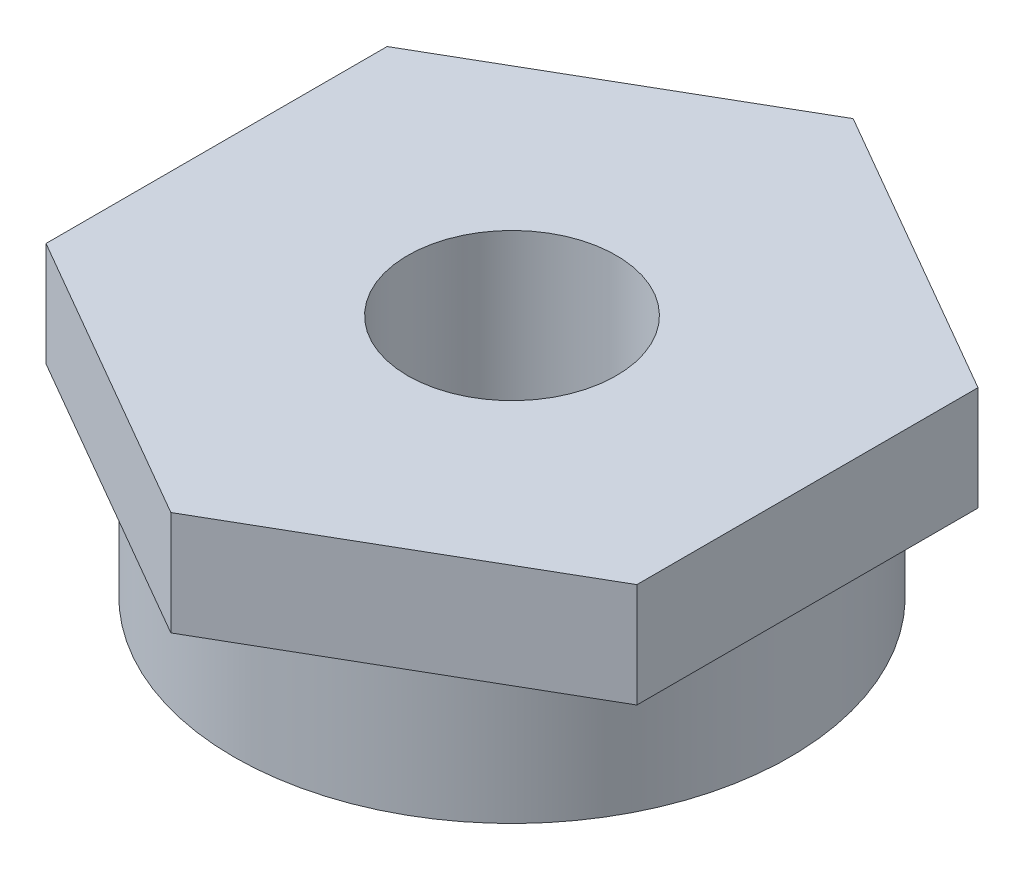
SolidWorks part; units mm, degrees
material "Q235A"
ref_plane "Front Plane" through (0, 0, 0) normal (0, 0, 1) x (1, 0, 0)
ref_plane "Top Plane" through (0, 0, 0) normal (0, 1, 0) x (1, 0, 0)
ref_plane "Right Plane" through (0, 0, 0) normal (1, 0, 0) x (0, 0, -1)
sketch "Sketch1" plane through (0, 0, 0) normal (0, 1, 0) x (1, 0, 0)
  circle A0 centre (0, 0) radius 4
  dimension "D1" = 8
extrude "Boss-Extrude1" add sketch "Sketch1" along normal blind 2
sketch "Sketch2" plane through (0, 2, 0) normal (0, 1, 0) x (1, 0, 0)
  line L1 (0, 4.9075) -> (-4.25, 2.4537)
  line L2 (-4.25, 2.4537) -> (-4.25, -2.4537)
  line L3 (-4.25, -2.4537) -> (0, -4.9075)
  line L4 (0, -4.9075) -> (4.25, -2.4537)
  line L5 (4.25, -2.4537) -> (4.25, 2.4537)
  line L6 (4.25, 2.4537) -> (0, 4.9075)
  circle A0 centre (0, 0) radius 4.25 construction
  dimension "D1" = 8.5
extrude "Boss-Extrude2" add sketch "Sketch2" along normal blind 1.5
sketch "Sketch3" plane through (0, 3.5, 0) normal (0, 1, 0) x (1, 0, 0)
  circle A0 centre (0, 0) radius 1.5
  dimension "D1" = 3
extrude "Cut-Extrude1" cut sketch "Sketch3" against normal through all
